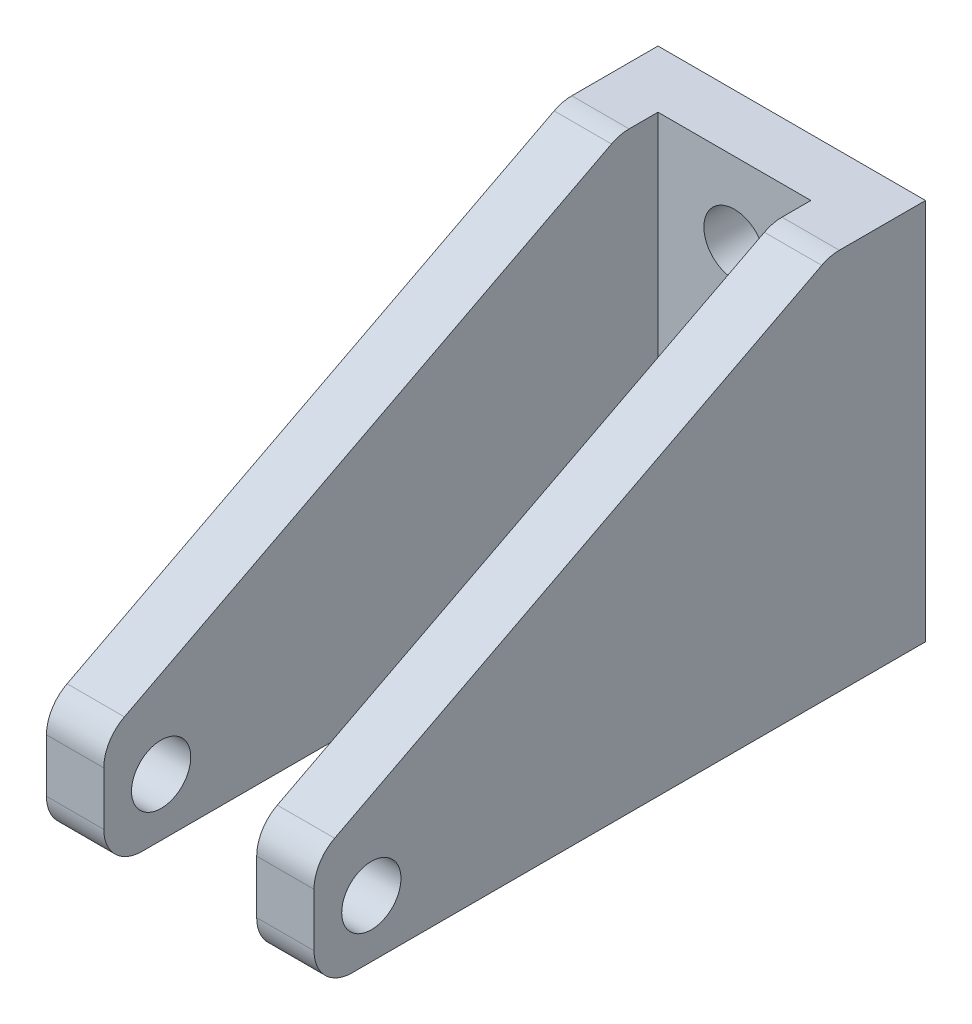
SolidWorks part; units mm, degrees
material "6061 合金"
ref_plane "前视基准面" through (0, 0, 0) normal (0, 0, 1) x (1, 0, 0)
ref_plane "上视基准面" through (0, 0, 0) normal (0, 1, 0) x (1, 0, 0)
ref_plane "右视基准面" through (0, 0, 0) normal (1, 0, 0) x (0, 0, -1)
other "Configuration Table"
sketch "草图1" plane through (0, 0, 0) normal (0, 1, 0) x (1, 0, 0)
  line L1 (-7, -16) -> (7, -16)
  line L2 (-7, -16) -> (-7, 16)
  line L3 (-7, 16) -> (7, 16)
  line L4 (7, -16) -> (7, 16)
  line L5 (-7, -16) -> (7, 16) construction
  line L6 (-7, 16) -> (7, -16) construction
  point P0 (0, 0)
  dimension "D1" = 14
  dimension "D2" = 32
extrude "凸台-拉伸1" add sketch "草图1" along normal blind 20
sketch "草图2" plane through (7, 0, 0) normal (1, 0, 0) x (0, 0, -1)
  line L0 (-16, 6) -> (11, 20)
  line L1 (-16, 20) -> (-16, 0) construction
  line L2 (-16, 20) -> (16, 20) construction
  line L3 (11, 20) -> (-16, 20)
  line L4 (-16, 20) -> (-16, 6)
  line L5 (-16, 0) -> (16, 0) construction
  line L6 (16, 20) -> (16, 0) construction
  dimension "D1" = 6
  dimension "D2" = 5
extrude "切除-拉伸1" cut sketch "草图2" against normal blind 20
sketch "草图3" plane through (0, 0, 0) normal (0, -1, 0) x (1, 0, 0)
  line L0 (-7, 16) -> (7, 16) construction
  line L1 (4, 16) -> (-4, 16)
  line L2 (4, 16) -> (4, -13)
  line L3 (4, -13) -> (-4, -13)
  line L4 (-4, 16) -> (-4, -13)
  line L5 (7, -16) -> (-7, -16) construction
  point P6 (0, 16)
  dimension "D1" = 8
  dimension "D2" = 3
extrude "切除-拉伸2" cut sketch "草图3" against normal blind 20
fillet "圆角2" radius 2 6 edges at (5.5, 20, -11) (5.5, 6, 16) (5.5, 0, 16) (-5.5, 0, 16) (-5.5, 20, -11) (-5.5, 6, 16)
sketch "草图4" plane through (-7, 0, 0) normal (-1, 0, 0) x (0, 0, 1)
  line L0 (-16, 0) -> (14, 0) construction
  line L1 (16, 4.7842) -> (16, 2) construction
  circle A0 centre (13, 3) radius 1.55
  dimension "D1" = 3.1
  dimension "D2" = 3
  dimension "D3" = 3
extrude "切除-拉伸3" cut sketch "草图4" against normal blind 20
sketch "草图5" plane through (0, 0, -13) normal (0, 0, 1) x (1, 0, 0)
  circle A0 centre (0, 16) radius 1.6
  circle A1 centre (0, 6) radius 1.6
  point P4 (0, 0)
  dimension "D1" = 3.2
  dimension "D2" = 3.2
  dimension "D3" = 10
  dimension "D4" = 6
extrude "切除-拉伸4" cut sketch "草图5" against normal blind 20
